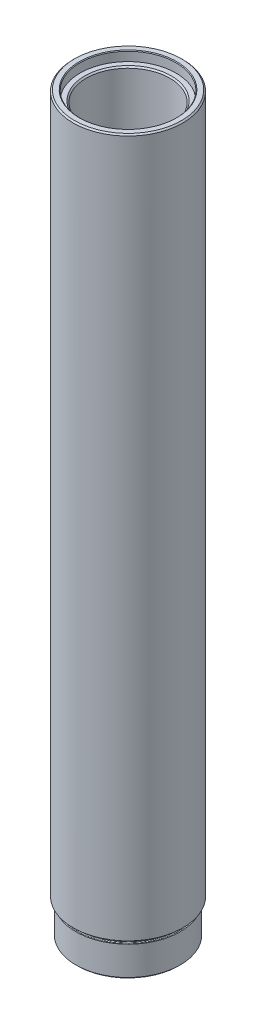
SolidWorks part; units mm, degrees
material "普通碳钢"
ref_plane "Front Plane" through (0, 0, 0) normal (0, 0, 1) x (1, 0, 0)
ref_plane "Top Plane" through (0, 0, 0) normal (0, 1, 0) x (1, 0, 0)
ref_plane "Right Plane" through (0, 0, 0) normal (1, 0, 0) x (0, 0, -1)
sketch "Sketch1" plane through (0, 0, 0) normal (0, 1, 0) x (1, 0, 0)
  circle A0 centre (0, 0) radius 30
  circle A1 centre (0, 0) radius 40
  dimension "D1" = 60
  dimension "D2" = 80
extrude "Boss-Extrude1" add sketch "Sketch1" along normal blind 537.5
sketch "Sketch2" plane through (0, 0, 0) normal (0, -1, 0) x (1, 0, 0)
  circle A0 centre (0, 0) radius 55.0291
  circle A1 centre (0, 0) radius 36.75
  dimension "D1" = 73.5
extrude "Cut-Extrude1" cut sketch "Sketch2" against normal blind 3 from offset 25 offset against normal yes
sketch "Sketch3" plane through (0, 0, 0) normal (0, -1, 0) x (1, 0, 0)
  circle A0 centre (0, 0) radius 38
  circle A1 centre (0, 0) radius 40
  dimension "D1" = 76
  dimension "D2" = 80
extrude "Cut-Extrude2" cut sketch "Sketch3" against normal blind 25
cosmetic thread "Cosmetic Thread1" parameters "D2"=73.7
chamfer "Chamfer1" distance 1 angle 45 2 edges at (0, 537.5, 40) (0, 0, -38)
sketch "Sketch4" plane through (0, 537.5, 0) normal (0, 1, 0) x (1, 0, 0)
  circle A0 centre (0, 0) radius 33.5751
extrude "Boss-Extrude2" add sketch "Sketch4" against normal blind 40
sketch "Sketch5" plane through (0, 537.5, 0) normal (0, 1, 0) x (1, 0, 0)
  circle A0 centre (0, 0) radius 25
  dimension "D1" = 50
extrude "Cut-Extrude3" cut sketch "Sketch5" against normal blind 6
sketch "Sketch6" plane through (0, 531.5, 0) normal (0, 1, 0) x (1, 0, 0)
  circle A0 centre (0, 0) radius 21.5
  dimension "D1" = 43
extrude "Cut-Extrude4" cut sketch "Sketch6" against normal through all
chamfer "Chamfer2" distance 1 angle 45 1 edges at (0, 531.5, 21.5)
sketch "Sketch9" plane through (0, 497.5, 0) normal (0, -1, 0) x (1, 0, 0)
  circle A1 centre (0, 0) radius 30
  circle A2 centre (0, 0) radius 30
  dimension "D1" = 0
extrude "Cut-Extrude7" cut sketch "Sketch9" against normal up to surface (40 mm away) up to face at (0, 537.5, 25)
sketch "Sketch10" plane through (0, 537.5, 0) normal (0, 1, 0) x (1, 0, 0)
  circle A0 centre (0, 0) radius 35
  dimension "D1" = 70
extrude "Cut-Extrude8" cut sketch "Sketch10" against normal blind 7
hole_wizard "M64x4.0 Tapped Hole1" positions "Sketch11" profile "Sketch12" tap size "M64x4.0" standard "GB"
sketch "Sketch11" plane through (0, 530.5, 0) normal (0, 1, 0) x (1, 0, 0)
  point P0 (0, 0)
sketch "Sketch12" plane through (0, 530.5, 0) normal (1, 0, 0) x (0, 0, 1)
  line L0 (0, 0) -> (0, 38.0258)
  line L1 (0, 38.0258) -> (30, 20)
  line L2 (30, 20) -> (30, 0)
  line L5 (30, 0) -> (0, 0)
  line L10 (0, 38.0258) -> (-30, 20) construction
  line L11 (0, -6.35) -> (0, 107.95) construction
  dimension "螺纹孔钻头直径" = 60
  dimension "螺纹孔钻头深度" = 20
  dimension "导头角度" = 118
chamfer "Chamfer3" distance 0.5 angle 45 1 edges at (0, 537.5, 35)
chamfer "Chamfer4" distance 0.5 angle 45 1 edges at (0, 530.5, 30)
sketch "Sketch13" plane through (0, 0, 0) normal (0, -1, 0) x (1, 0, 0)
  circle A1 centre (0, 0) radius 40
  circle A2 centre (0, 0) radius 40
  dimension "D1" = 0
extrude "Cut-Extrude9" cut sketch "Sketch13" against normal blind 3
chamfer "Chamfer5" distance 1 angle 45 1 edges at (0, 3, -38)
chamfer "Chamfer7" distance 0.5 angle 45 1 edges at (0, 28, -40)
fillet "Fillet1" radius 0.5 2 edges at (0, 25, -36.75) (0, 28, -36.75)
hole_wizard "M64x3.0 Tapped Hole1" positions "Sketch14" profile "Sketch15" tap size "M64x3.0" standard "DIN"
sketch "Sketch14" plane through (0, 530.5, 0) normal (0, 1, 0) x (1, 0, 0)
  point P0 (0, 0)
sketch "Sketch15" plane through (0, 530.5, 0) normal (1, 0, 0) x (0, 0, 1)
  line L0 (0, 0) -> (0, 73.3262)
  line L1 (0, 73.3262) -> (30.5, 55)
  line L2 (30.5, 55) -> (30.5, 0)
  line L5 (30.5, 0) -> (0, 0)
  line L10 (0, 73.3262) -> (-30.5, 55) construction
  line L11 (0, -6.35) -> (0, 107.95) construction
  dimension "螺纹孔钻头直径" = 61
  dimension "螺纹孔钻头深度" = 55
  dimension "导头角度" = 118
cosmetic thread "孔螺蚊线1" parameters "D1"=40, "D2"=64
chamfer "Chamfer8" distance 1 angle 45 1 edges at (0, 530.5, 30.5)
